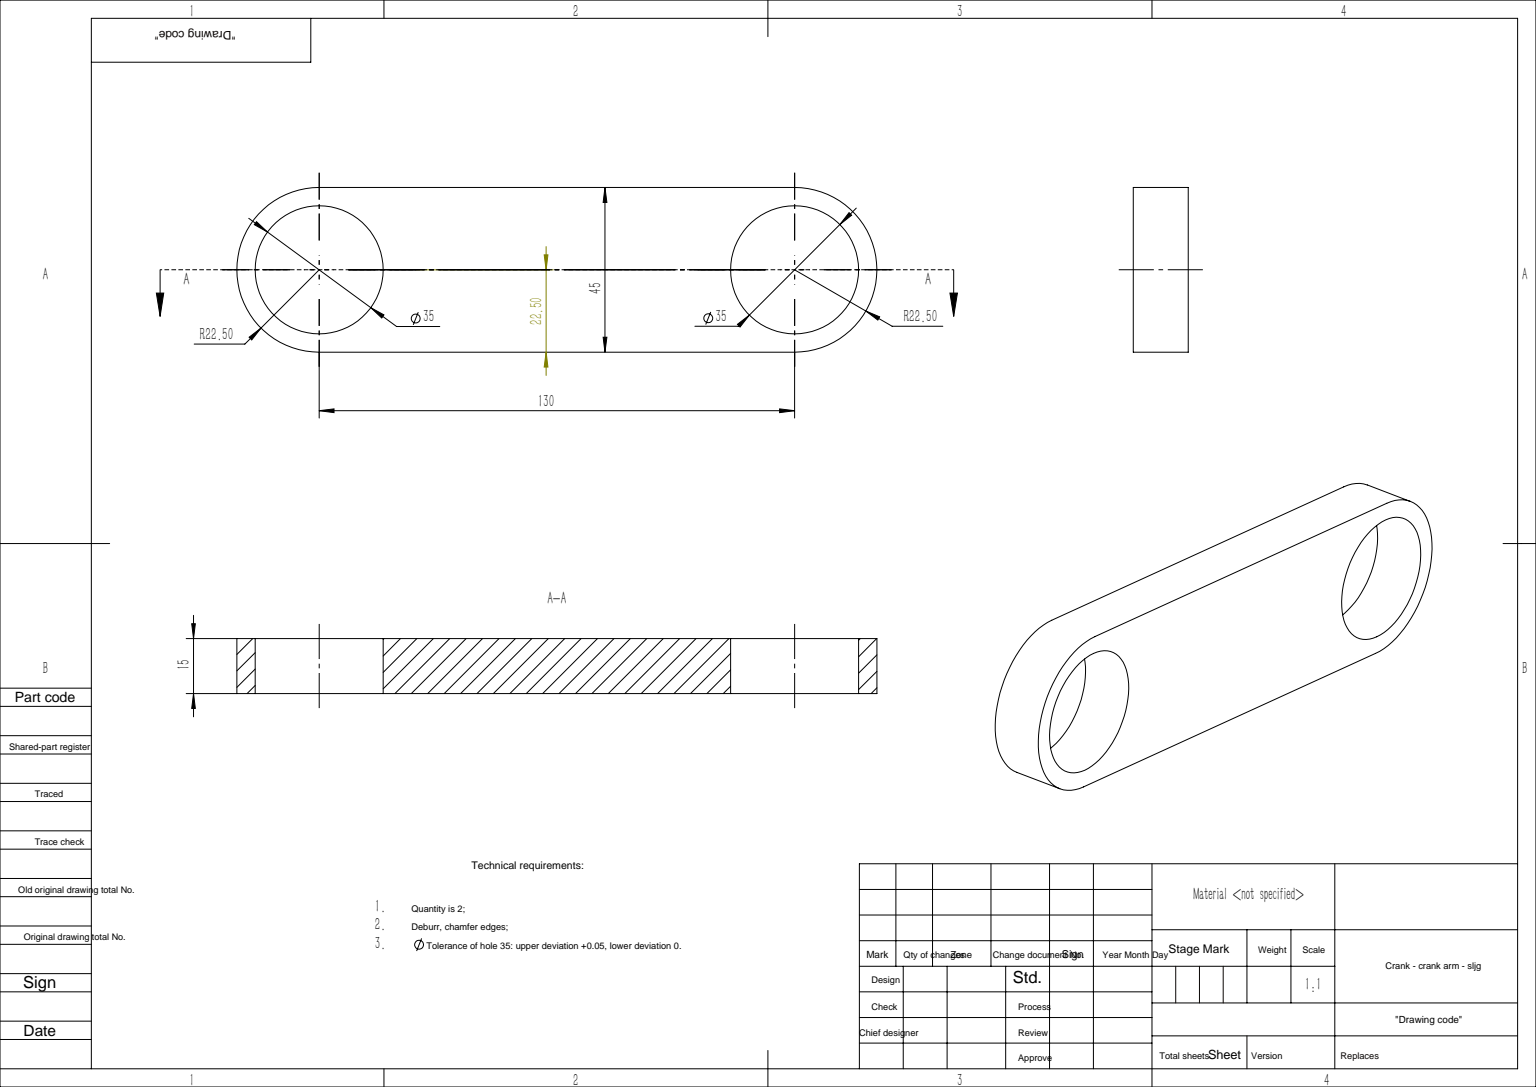
SolidWorks part; units mm, degrees
ref_plane "前视基准面" through (0, 0, 0) normal (0, 0, 1) x (1, 0, 0)
ref_plane "上视基准面" through (0, 0, 0) normal (0, 1, 0) x (1, 0, 0)
ref_plane "右视基准面" through (0, 0, 0) normal (1, 0, 0) x (0, 0, -1)
sketch "草图1" plane through (0, 0, 0) normal (1, 0, 0) x (0, 0, -1)
  line L0 (0, 0) -> (0, -130) construction
  line L1 (22.5, 0) -> (22.5, -130)
  line L2 (-22.5, 0) -> (-22.5, -130)
  arc A0 (22.5, 0) -> (-22.5, 0) centre (0, 0) ccw
  arc A1 (-22.5, -130) -> (22.5, -130) centre (0, -130) ccw
  point P3 (0, -65)
  dimension "D1" = 22.5
  dimension "D2" = 130
extrude "凸台-拉伸1" add sketch "草图1" along normal blind 15 contours A0 L2 A1 L1
sketch "草图2" plane through (15, 0, 0) normal (1, 0, 0) x (0, 0, -1)
  circle A0 centre (0, 0) radius 17.5
  dimension "D1" = 35
extrude "切除-拉伸1" cut sketch "草图2" against normal through all
sketch "草图3" plane through (0, 0, 0) normal (-1, 0, 0) x (0, 0, 1)
  circle A0 centre (0, -130) radius 17.5
  dimension "D1" = 35
extrude "切除-拉伸2" cut sketch "草图3" against normal through all
